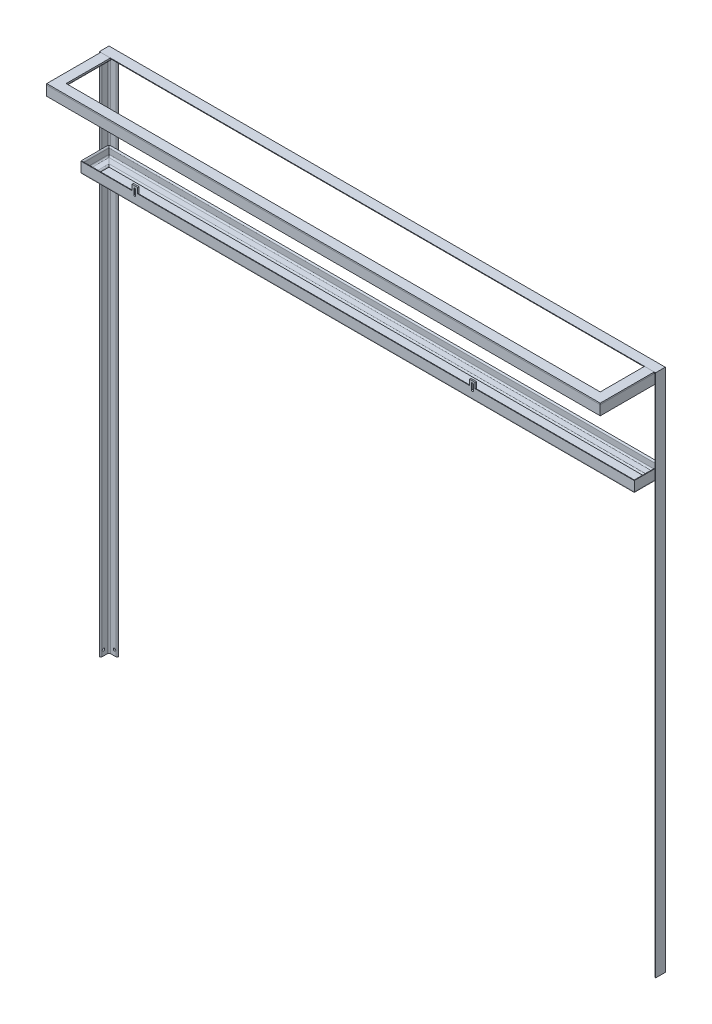
from build123d import *

# Parameters (mm, degrees)
MEMBER_1_DEPTH        = 1944.497474683
MEMBER_1_2_DEPTH      = 2060.497474683
MEMBER_1_2_DEPTH_BACK = 50.497474683
MEMBER_1_3_DEPTH      = 1944.497474683
MEMBER_2_DEPTH        = 275.497474683
MEMBER_2_2_DEPTH      = 2100.994949366
MEMBER_2_3_DEPTH      = 275.497474683
MEMBER_3_DEPTH        = 152.497474683
MEMBER_3_DEPTH_BACK   = 50.497474683
MEMBER_3_2_DEPTH      = 2100.994949366
MEMBER_3_3_DEPTH      = 202.994949366
MEMBER_3_4_DEPTH      = 2100.994949366
SKETCH_8_R            = 4.5
CUT_EXTRUDE_1_DEPTH   = 10
SKETCH_9_R            = 4.5
CUT_EXTRUDE_2_DEPTH   = 697
EXTRUDE_1_DEPTH       = 5
EXTRUDE_2_DEPTH       = 2
SKETCH_13_W           = 20
SKETCH_13_H           = 30
EXTRUDE_3_DEPTH       = 5
CUT_EXTRUDE_3_DEPTH   = 10


with BuildPart() as part:
    # Sketch1 on segment 1 (carried to segment 1) → Member 1 (new body)
    with BuildSketch(Plane.ZX.offset(-1894)):
        with BuildLine():
            Line((0, 0), (0, 35))
            ThreePointArc((0, 35), (3.535533906, 33.535533906), (5, 30))
            Line((5, 30), (5, 10))
            ThreePointArc((5, 10), (6.464466094, 6.464466094), (10, 5))
            Line((10, 5), (30, 5))
            ThreePointArc((30, 5), (33.535533906, 3.535533906), (35, 0))
            Line((35, 0), (0, 0))
        make_face()
    extrude(amount=MEMBER_1_DEPTH)

    # Member 1 mitre 1
    split(bisect_by=Plane(origin=(0, 0, 0), x_dir=(0.707106781, -0.707106781, 0), z_dir=(-0.707106781, -0.707106781, 0)), keep=Keep.TOP)


with BuildPart() as body_2:
    # Sketch1 → Member 1 2 (new, two sides: drawn at the far end of the back side and taken through both)
    with BuildSketch(Plane(origin=(0, 0, 0), x_dir=(0, 0, 1), z_dir=(1, 0, 0)).offset(-MEMBER_1_2_DEPTH_BACK)):
        with BuildLine():
            Line((0, 0), (0, 35))
            ThreePointArc((0, 35), (3.535533906, 33.535533906), (5, 30))
            Line((5, 30), (5, 10))
            ThreePointArc((5, 10), (6.464466094, 6.464466094), (10, 5))
            Line((10, 5), (30, 5))
            ThreePointArc((30, 5), (33.535533906, 3.535533906), (35, 0))
            Line((35, 0), (0, 0))
        make_face()
    extrude(amount=MEMBER_1_2_DEPTH + MEMBER_1_2_DEPTH_BACK)

    # Member 1 2 mitre 1
    split(bisect_by=Plane(origin=(0, 0, 0), x_dir=(-0.707106781, 0.707106781, 0), z_dir=(0.707106781, 0.707106781, 0)), keep=Keep.TOP)

    # Member 1 2 mitre 2
    split(bisect_by=Plane(origin=(2010, 0, 0), x_dir=(-0.707106781, -0.707106781, 0), z_dir=(-0.707106781, 0.707106781, 0)), keep=Keep.TOP)


with BuildPart() as body_3:
    # Sketch1 on segment 3 (carried to segment 3) → Member 1 3 (new body)
    with BuildSketch(Plane(origin=(2010, 50.497474683, 0), x_dir=(0, 0, 1), z_dir=(0, -1, 0))):
        with BuildLine():
            Line((0, 0), (0, 35))
            ThreePointArc((0, 35), (3.535533906, 33.535533906), (5, 30))
            Line((5, 30), (5, 10))
            ThreePointArc((5, 10), (6.464466094, 6.464466094), (10, 5))
            Line((10, 5), (30, 5))
            ThreePointArc((30, 5), (33.535533906, 3.535533906), (35, 0))
            Line((35, 0), (0, 0))
        make_face()
    extrude(amount=MEMBER_1_3_DEPTH)

    # Member 1 3 mitre 1
    split(bisect_by=Plane(origin=(2010, 0, 0), x_dir=(0.707106781, 0.707106781, 0), z_dir=(0.707106781, -0.707106781, 0)), keep=Keep.TOP)


with BuildPart() as body_4:
    # Sketch11 → Member 2 (new body)
    with BuildSketch(Plane(origin=(5, -5, 5), x_dir=(0, -1, 0), z_dir=(0, 0, 1))):
        with BuildLine():
            Line((0, 0), (0, 35))
            ThreePointArc((0, 35), (3.535533906, 33.535533906), (5, 30))
            Line((5, 30), (5, 10))
            ThreePointArc((5, 10), (6.464466094, 6.464466094), (10, 5))
            Line((10, 5), (30, 5))
            ThreePointArc((30, 5), (33.535533906, 3.535533906), (35, 0))
            Line((35, 0), (0, 0))
        make_face()
    extrude(amount=MEMBER_2_DEPTH)

    # Member 2 mitre 1
    split(bisect_by=Plane(origin=(5, -5, 230), x_dir=(0, -1, 0), z_dir=(-0.707106781, 0, -0.707106781)), keep=Keep.TOP)


with BuildPart() as body_5:
    # Sketch11 on segment 2 (carried to segment 2) → Member 2 2 (new body)
    with BuildSketch(Plane(origin=(-45.497474683, -5, 230), x_dir=(0, -1, 0), z_dir=(1, 0, 0))):
        with BuildLine():
            Line((0, 0), (0, 35))
            ThreePointArc((0, 35), (3.535533906, 33.535533906), (5, 30))
            Line((5, 30), (5, 10))
            ThreePointArc((5, 10), (6.464466094, 6.464466094), (10, 5))
            Line((10, 5), (30, 5))
            ThreePointArc((30, 5), (33.535533906, 3.535533906), (35, 0))
            Line((35, 0), (0, 0))
        make_face()
    extrude(amount=MEMBER_2_2_DEPTH)

    # Member 2 2 mitre 1
    split(bisect_by=Plane(origin=(2005, -5, 230), x_dir=(0, -1, 0), z_dir=(-0.707106781, 0, 0.707106781)), keep=Keep.TOP)

    # Member 2 2 mitre 2
    split(bisect_by=Plane(origin=(5, -5, 230), x_dir=(0, 1, 0), z_dir=(0.707106781, 0, 0.707106781)), keep=Keep.TOP)


with BuildPart() as body_6:
    # Sketch11 on segment 3 (carried to segment 3) → Member 2 3 (new body)
    with BuildSketch(Plane(origin=(2005, -5, 280.497474683), x_dir=(0, -1, 0), z_dir=(0, 0, -1))):
        with BuildLine():
            Line((0, 0), (0, 35))
            ThreePointArc((0, 35), (3.535533906, 33.535533906), (5, 30))
            Line((5, 30), (5, 10))
            ThreePointArc((5, 10), (6.464466094, 6.464466094), (10, 5))
            Line((10, 5), (30, 5))
            ThreePointArc((30, 5), (33.535533906, 3.535533906), (35, 0))
            Line((35, 0), (0, 0))
        make_face()
    extrude(amount=MEMBER_2_3_DEPTH)

    # Member 2 3 mitre 1
    split(bisect_by=Plane(origin=(2005, -5, 230), x_dir=(0, 1, 0), z_dir=(0.707106781, 0, -0.707106781)), keep=Keep.TOP)


with BuildPart() as body_7:
    # Sketch12 → Member 3 (new, two sides: drawn at the far end of the back side and taken through both)
    with BuildSketch(Plane(origin=(2005, -339, 5), x_dir=(0, 1, 0), z_dir=(0, 0, 1)).offset(-MEMBER_3_DEPTH_BACK)):
        with BuildLine():
            Line((0, 0), (0, 35))
            ThreePointArc((0, 35), (3.535533906, 33.535533906), (5, 30))
            Line((5, 30), (5, 10))
            ThreePointArc((5, 10), (6.464466094, 6.464466094), (10, 5))
            Line((10, 5), (30, 5))
            ThreePointArc((30, 5), (33.535533906, 3.535533906), (35, 0))
            Line((35, 0), (0, 0))
        make_face()
    extrude(amount=MEMBER_3_DEPTH + MEMBER_3_DEPTH_BACK)

    # Member 3 mitre 1
    split(bisect_by=Plane(origin=(2005, -339, 5), x_dir=(0, 1, 0), z_dir=(0.707106781, 0, 0.707106781)), keep=Keep.TOP)

    # Member 3 mitre 2
    split(bisect_by=Plane(origin=(2005, -339, 107), x_dir=(0, 1, 0), z_dir=(0.707106781, 0, -0.707106781)), keep=Keep.TOP)


with BuildPart() as body_8:
    # Sketch12 on segment 2 (carried to segment 2) → Member 3 2 (new body)
    with BuildSketch(Plane(origin=(2055.497474683, -339, 107), x_dir=(0, 1, 0), z_dir=(-1, 0, 0))):
        with BuildLine():
            Line((0, 0), (0, 35))
            ThreePointArc((0, 35), (3.535533906, 33.535533906), (5, 30))
            Line((5, 30), (5, 10))
            ThreePointArc((5, 10), (6.464466094, 6.464466094), (10, 5))
            Line((10, 5), (30, 5))
            ThreePointArc((30, 5), (33.535533906, 3.535533906), (35, 0))
            Line((35, 0), (0, 0))
        make_face()
    extrude(amount=MEMBER_3_2_DEPTH)

    # Member 3 2 mitre 1
    split(bisect_by=Plane(origin=(2005, -339, 107), x_dir=(0, -1, 0), z_dir=(-0.707106781, 0, 0.707106781)), keep=Keep.TOP)

    # Member 3 2 mitre 2
    split(bisect_by=Plane(origin=(5, -339, 107), x_dir=(0, 1, 0), z_dir=(0.707106781, 0, 0.707106781)), keep=Keep.TOP)

    # 草图13 → 凸台-拉伸3 (add)
    with BuildSketch(Plane.XY.offset(107)):
        with Locations((200, -299)):
            Rectangle(SKETCH_13_W, SKETCH_13_H)
        with Locations((1420, -299)):
            Rectangle(SKETCH_13_W, SKETCH_13_H)
    extrude(amount=-EXTRUDE_3_DEPTH)

    # 草图12 → 切除-拉伸3 (cut)
    with BuildSketch(Plane.XY.offset(107)):
        with BuildLine():
            Line((196.5, -294), (196.5, -314))
            ThreePointArc((196.5, -314), (200, -317.5), (203.5, -314))
            Line((203.5, -314), (203.5, -294))
            ThreePointArc((203.5, -294), (200, -290.5), (196.5, -294))
        make_face()
        with BuildLine():
            Line((1416.5, -294), (1416.5, -314))
            ThreePointArc((1416.5, -314), (1420, -317.5), (1423.5, -314))
            Line((1423.5, -314), (1423.5, -294))
            ThreePointArc((1423.5, -294), (1420, -290.5), (1416.5, -294))
        make_face()
    extrude(amount=-CUT_EXTRUDE_3_DEPTH, mode=Mode.SUBTRACT)


with BuildPart() as body_9:
    # Sketch12 on segment 3 (carried to segment 3) → Member 3 3 (new body)
    with BuildSketch(Plane(origin=(5, -339, 157.497474683), x_dir=(0, 1, 0), z_dir=(0, 0, -1))):
        with BuildLine():
            Line((0, 0), (0, 35))
            ThreePointArc((0, 35), (3.535533906, 33.535533906), (5, 30))
            Line((5, 30), (5, 10))
            ThreePointArc((5, 10), (6.464466094, 6.464466094), (10, 5))
            Line((10, 5), (30, 5))
            ThreePointArc((30, 5), (33.535533906, 3.535533906), (35, 0))
            Line((35, 0), (0, 0))
        make_face()
    extrude(amount=MEMBER_3_3_DEPTH)

    # Member 3 3 mitre 1
    split(bisect_by=Plane(origin=(5, -339, 107), x_dir=(0, -1, 0), z_dir=(-0.707106781, 0, -0.707106781)), keep=Keep.TOP)

    # Member 3 3 mitre 2
    split(bisect_by=Plane(origin=(5, -339, 5), x_dir=(0, -1, 0), z_dir=(-0.707106781, 0, 0.707106781)), keep=Keep.TOP)


with BuildPart() as body_10:
    # Sketch12 on segment 4 (carried to segment 4) → Member 3 4 (new body)
    with BuildSketch(Plane(origin=(-45.497474683, -339, 5), x_dir=(0, 1, 0), z_dir=(1, 0, 0))):
        with BuildLine():
            Line((0, 0), (0, 35))
            ThreePointArc((0, 35), (3.535533906, 33.535533906), (5, 30))
            Line((5, 30), (5, 10))
            ThreePointArc((5, 10), (6.464466094, 6.464466094), (10, 5))
            Line((10, 5), (30, 5))
            ThreePointArc((30, 5), (33.535533906, 3.535533906), (35, 0))
            Line((35, 0), (0, 0))
        make_face()
    extrude(amount=MEMBER_3_4_DEPTH)

    # Member 3 4 mitre 1
    split(bisect_by=Plane(origin=(2005, -339, 5), x_dir=(0, -1, 0), z_dir=(-0.707106781, 0, -0.707106781)), keep=Keep.TOP)

    # Member 3 4 mitre 2
    split(bisect_by=Plane(origin=(5, -339, 5), x_dir=(0, 1, 0), z_dir=(0.707106781, 0, -0.707106781)), keep=Keep.TOP)


with BuildPart() as cut_extrude_1_tool:
    # 草图8 → 切除-拉伸1 (new body)
    with BuildSketch(Plane.XY.offset(5)):
        with Locations((25, -1874)):
            Circle(SKETCH_8_R)
        with Locations((1985, -1874)):
            Circle(SKETCH_8_R)
    extrude(amount=-CUT_EXTRUDE_1_DEPTH)


with BuildPart() as part_1:
    add(part.part)

    # 切除-拉伸1: cut by cut_extrude_1_tool
    add(cut_extrude_1_tool.part, mode=Mode.SUBTRACT)

    # 草图9 → 切除-拉伸2 (cut)
    with BuildSketch(Plane.ZY):
        with Locations((25, -1874)):
            Circle(SKETCH_9_R)
    extrude(amount=-CUT_EXTRUDE_2_DEPTH, mode=Mode.SUBTRACT)


with BuildPart() as body_3_1:
    add(body_3.part)

    # 切除-拉伸1: cut by cut_extrude_1_tool
    add(cut_extrude_1_tool.part, mode=Mode.SUBTRACT)


with BuildPart() as body_11:
    # 草图10 → 凸台-拉伸1 (new body)
    with BuildSketch(Plane(origin=(0, -5, 0), x_dir=(1, 0, 0), z_dir=(0, 1, 0))):
        Polygon((5, -35), (5, -230), (2005, -230), (2005, -35), (1970, -35), (1970, -195), (40, -195), (40, -35), align=None)
    extrude(amount=EXTRUDE_1_DEPTH)


with BuildPart() as body_12:
    # 草图11 → 凸台-拉伸2 (new body)
    with BuildSketch(Plane.XZ.offset(339)):
        with BuildLine():
            Line((5, 107), (2005, 107))
            Line((2005, 107), (2005, 10))
            ThreePointArc((2005, 10), (2003.535533906, 6.464466094), (2000, 5))
            Line((2000, 5), (10, 5))
            ThreePointArc((10, 5), (6.464466094, 6.464466094), (5, 10))
            Line((5, 10), (5, 107))
        make_face()
    extrude(amount=EXTRUDE_2_DEPTH)


solid = Compound([body_2.part, body_4.part, body_5.part, body_6.part, body_7.part, body_8.part, body_9.part, body_10.part, part_1.part, body_3_1.part, body_11.part, body_12.part])
